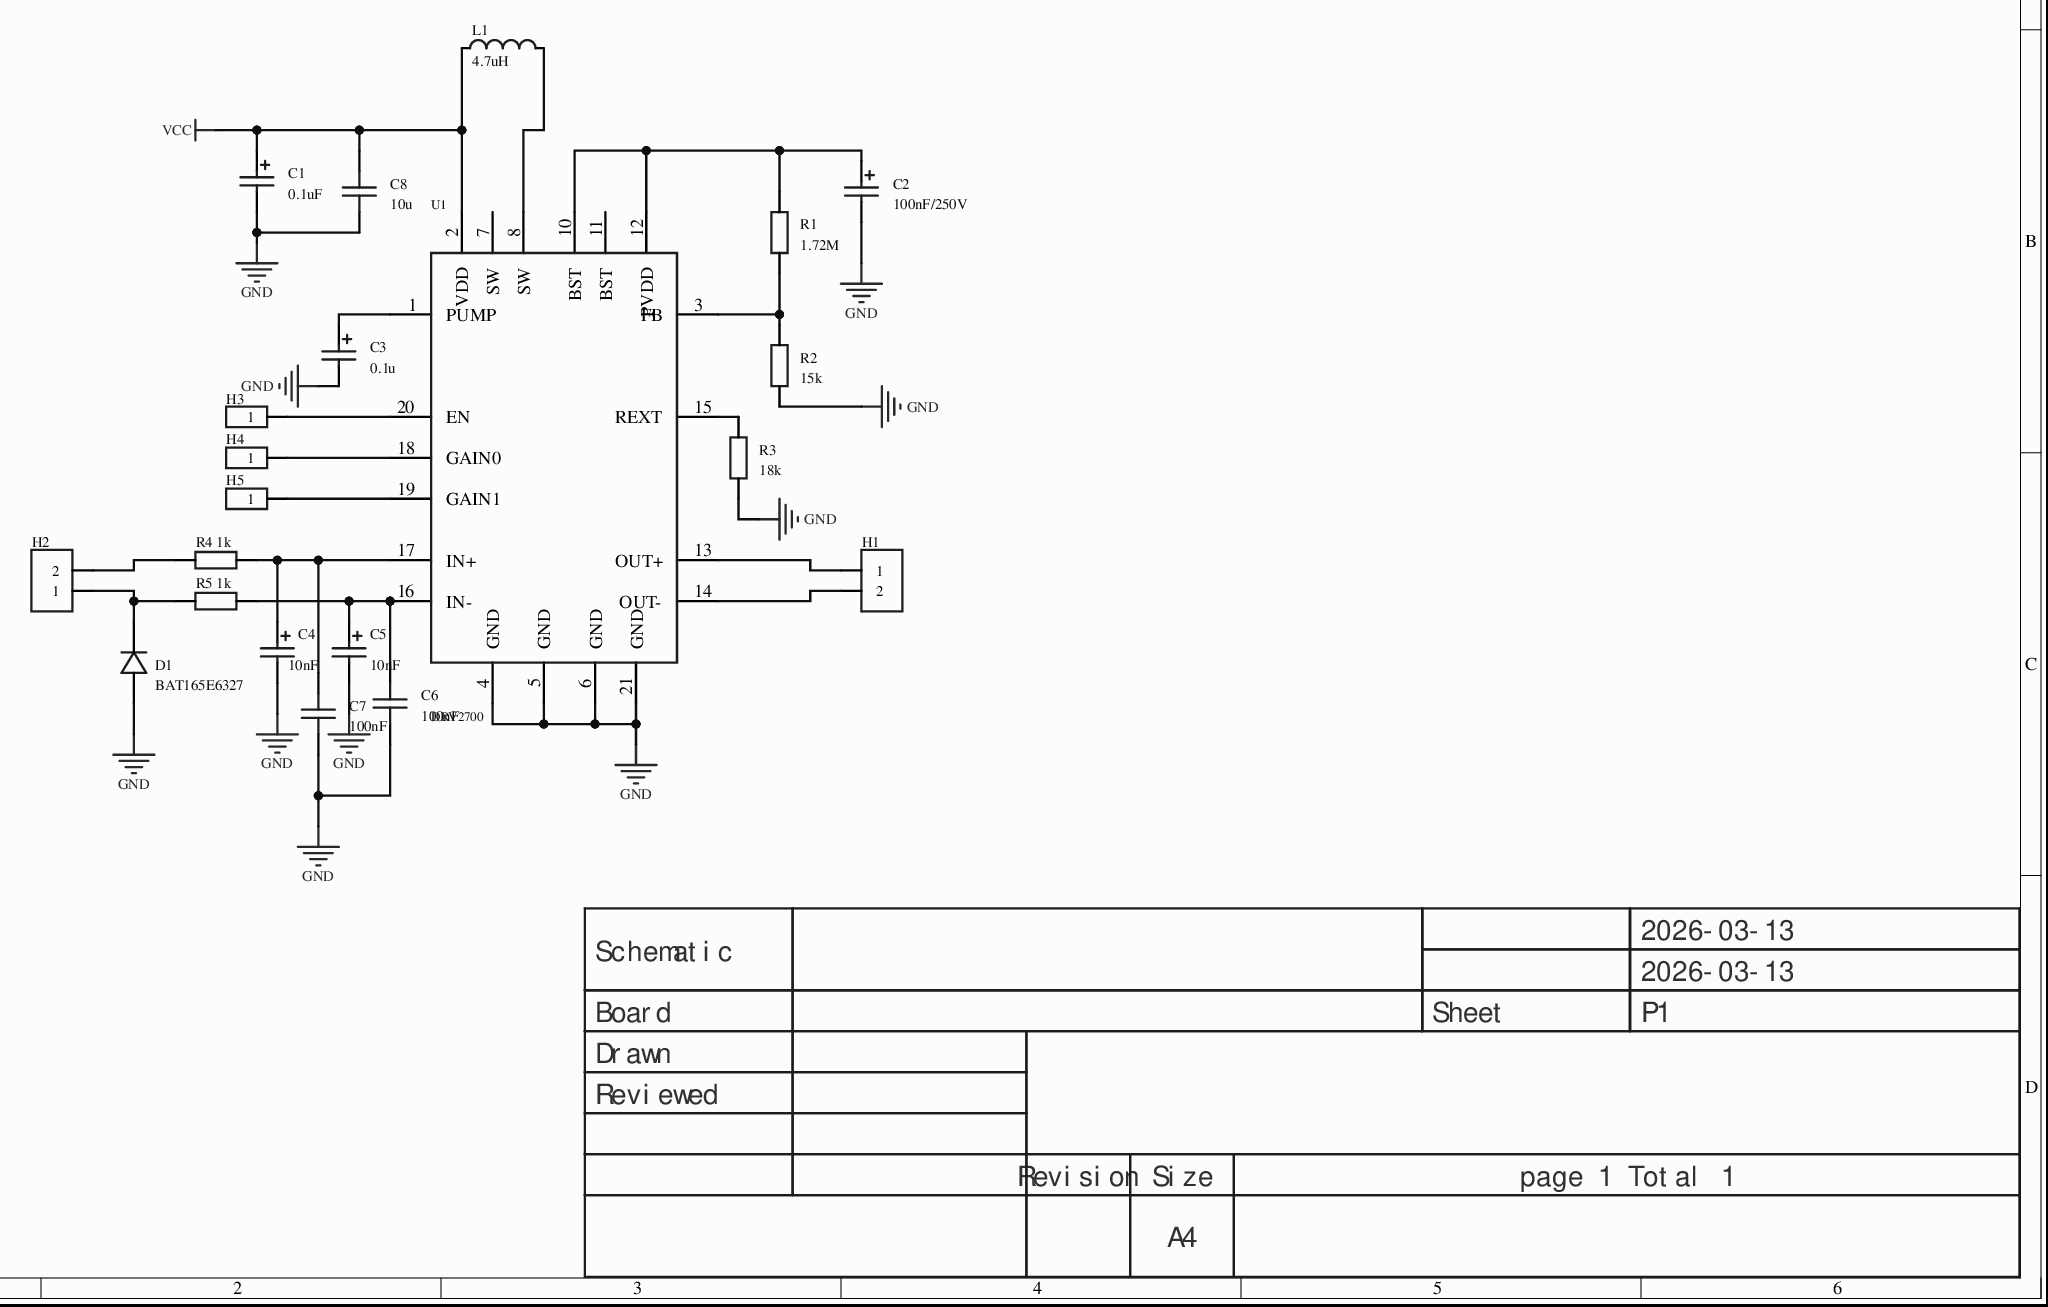
[diagram p0: MISC51187-3.schdoc]
# Altium project MISC51187-2.PrjPcb
1 sheet, 21 parts. Net scope: global (net labels, ports and power ports of the same name join across sheets).
Board file: MISC51187.pcbdoc

## Sheet MISC51187-3.schdoc
size 297 x 209 mm; Version: V1.0; @Project Name: MISC51187; @Update Date: 2026-03-13; @Create Date: 2026-03-13; @Board Name: MISC51187; @Create Time: 10:06:33; @Page Count: 1; @Page No: 1; @Schematic Name: MISC51187; @Update Time: 10:06:33; Size: A4

### Parts
C1  0.1uF  [C_Ele_SMD_3x5.4mm]
C2  100nF/250V  [C_Ele_SMD_3x5.4mm]
C3  0.1u  [C_Ele_SMD_3x5.4mm]
C4  10nF  [C_Ele_SMD_3x5.4mm]
C5  10nF  [C_Ele_SMD_3x5.4mm]
C6  100nF  [C0805]
C7  100nF  [C0805]
C8  10u  [C0805]
D1  BAT165E6327  [SOD-323_L1.8-W1.3-LS2.5-RD]
H1  (no value)  [HDR-TH_2P-P2.54-V-F]
H2  (no value)  [HDR-TH_2P-P2.54-V-F]
H3  (no value)  [HDR-TH_1P-V-M_XKB_X4611WV-01I-C28D40]
H4  (no value)  [HDR-TH_1P-V-M_XKB_X4611WV-01I-C28D40]
H5  (no value)  [HDR-TH_1P-V-M_XKB_X4611WV-01I-C28D40]
L1  4.7uH  [IND-SMD_L4.6-W4.1-A]
R1  1.72M  [Res_1W]
R2  15k  [Res_1W]
R3  18k  [Res_1/4W]
R4  1k  [Res_1/4W]
R5  1k  [Res_1/4W]
U1  DRV2700  [TI-RGP20-2700X2700TP_V]

### Nets
GND: C1.2 C2.2 C3.2 C4.2 C5.2 C6.1 C7.1 C8.1 D1.2(A) R2.1 R3.1 U1.4(GND) U1.5(GND) U1.6(GND) U1.21(GND)
VCC: C1.1 C8.2 L1.1 U1.2(VDD)
NetC2_1: C2.1 R1.2 U1.10(BST) U1.12(PVDD)
NetC3_1: C3.1 U1.1(PUMP)
NetC4_1: C4.1 C7.2 R4.2 U1.17(IN+)
NetC5_1: C5.1 C6.2 R5.2 U1.16(IN-)
NetD1_1: D1.1(C) H2.1 R5.1
NetH1_1: H1.1 U1.13(OUT+)
NetH1_2: H1.2 U1.14(OUT-)
NetH2_2: H2.2 R4.1
NetH3_1: H3.1 U1.20(EN)
NetH4_1: H4.1 U1.18(GAIN0)
NetH5_1: H5.1 U1.19(GAIN1)
NetL1_2: L1.2 U1.8(SW)
NetR1_1: R1.1 R2.2 U1.3(FB)
NetR3_2: R3.2 U1.15(REXT)

Not connected (* = marked no-connect by the designer): U1 7(SW)* 11(BST)*

### Notes on the sheet
- 2026-03-13
- Schematic
- Board
- Sheet
- P1
- Drawn
- Reviewed
- Revision
- Size
- A4
- page 1 Total 1

### Library data of the parts
C1-C5 = C_Ele_SMD_3x5.4mm: Symbol: CAP; 3D Model: 0132c3d3fdbf4fd987f710a97e7a5b5d0819f05c4eef4c71ace90d822a990e87; 3D Model Transform: 129.9,149.58,209.06,-90,0,0,0,0,0; AddInBom: yes; ModelName: CAP-SMD_BD3.0-L3.3-W3.3-H5.3; Device: C_Ele_SMD_3x5.4mm; Supplier Footprint: SMD,3x5.4mm; FootprintName: C_Ele_SMD_3x5.4mm; ConvertToPcb: yes
  C1: Value: 0.1uF
  C2: Value: 100nF/250V
  C3: Value: 0.1u
  C4 C5: Value: 10nF
C6-C8 = CAP_0805: Symbol: Capacitance; 3D Model: 1ba041120af144c991958decab20d2410819f05c4eef4c71ace90d822a990e87; 3D Model Transform: 78.74,51.181,0,0,0,0,0,0.0005,0; ConvertToPcb: yes; ModelName: C0805_L2.0-W1.3-H1.3; Device: CAP_0805; Supplier Footprint: 0805; FootprintName: C0805; AddInBom: yes
  C6 C7: Value: 100nF
  C8: Value: 10u
D1 = BAT165E6327: component BAT165E6327 compon Diode configuration: 1 single; Forward voltage (Vf): 740mV@750mA; DC reverse voltage (Vr): 40V; Rectifier current: 750mA;; Manufacturer: Infineon(英飞凌); Symbol: BAT165E6327HTSA1; Reverse Leakage Current (Ir): 50uA@40V; Non-Repetitive Peak Forward Surge Current: 2.5A; 3D Model: 7459fe65e23146c0a8d836e46a0add720819f05c4eef4c71ace90d822a990e87; 3D Model Transform: 104.3305,51.181,0,0,0,0,0,0,0; AddInBom: yes; Device: BAT165E6327; LCSC Part Name: 电压:40V 电流:750mA; Supplier Part: C151511; Manufacturer Part: BAT165E6327; Supplier Footprint: SOD-323; JLCPCB Part Class: Extended Part; Datasheet: https://item.szlcsc.com/datasheet/BAT165E6327/162851.html; Supplier: LCSC; Diode Configuration: 1 single; Voltage - Forward(Vf@If): 740mV@750mA; Voltage - DC Reverse(Vr): 40V; Current - Rectified: 750mA; FootprintName: SOD-323_L1.8-W1.3-LS2.5-RD; ConvertToPcb: yes; ModelName: SOD-323_L1.8-W1.3-LS2.5-RD
H1 H2 = HDR-F_2.54_1x2P: Symbol: Header-Female-2.54_1x2; 3D Model: a9450ef445564560a104363b9aacde4e0819f05c4eef4c71ace90d822a990e87; 3D Model Transform: 215.7476,98.425,0,0,0,0,0,0,-129.921; ConvertToPcb: yes; ModelName: HDR-TH_2P-P2.54-F-LI-1X2P; Device: HDR-F_2.54_1x2P; Supplier Part: C49661; Supplier Footprint: 插件; FootprintName: HDR-TH_2P-P2.54-V-F; AddInBom: yes
H3-H5 = HDR-M_2.54_1x1P: Symbol: HDR_1x1; 3D Model: 95857080d3cc4057a19a22ccce05e1710819f05c4eef4c71ace90d822a990e87; 3D Model Transform: 78.74,79.1337,0,0,0,0,0,0,-110.236; ConvertToPcb: yes; Device: HDR-M_2.54_1x1P; Supplier Part: C81276; Supplier Footprint: 插件; JLCPCB Part Class: Extended Part; FootprintName: HDR-TH_1P-V-M_XKB_X4611WV-01I-C28D40; AddInBom: yes; ModelName: HDR-TH_1P-V-M_XKB_X4611WV-01I-C28D40
L1 = SRG0420-4R7-M: component SRG0420-4R7-M comp Inductance: 4.7uH; Tolerance: ±20%; Rated current: 3A; Saturation current (Isat): 3.5A; Type: molded inductor;; Manufacturer: JIERR(捷而瑞); DC Resistance(DCR): 105mΩ; 3D Model: 3b00517e351145dc8b8e2e52a7e5ed2c0819f05c4eef4c71ace90d822a990e87; 3D Model Transform: 181.102,161.417,0,0,0,0,0,0,0; AddInBom: yes; ModelName: IND-SMD_L4.6-W4.1-H1.5; Symbol: SRG0420-4R7-M; Device: SRG0420-4R7-M; LCSC Part Name: 4.7μH ±20% 3.5A; Supplier Part: C53462918; Manufacturer Part: SRG0420-4R7-M; Supplier Footprint: SMD,4.6x4.1mm; JLCPCB Part Class: Extended Part; Datasheet: https://item.szlcsc.com/datasheet/SRG0420-4R7-M/56628163.html; Supplier: LCSC; Value: 4.7uH; Current Rating: 3A; Current - Saturation(Isat): 3.5A; Type: Molded inductor; FootprintName: IND-SMD_L4.6-W4.1-A; ConvertToPcb: yes
R1-R5 = Res_AXIAL-1W: Symbol: Resistor; 3D Model: f1f7cfb3d56f4763951150e77c261d090819f05c4eef4c71ace90d822a990e87; 3D Model Transform: 641.71,177.16,374,0,0,0,0,0,-190; ConvertToPcb: yes; ModelName: RES-TH_BD4.5-L11.5-P15.50-D0.8; Device: Res_AXIAL-1W; Supplier Footprint: 轴向引线; AddInBom: yes
  R1: Value: 1.72M; FootprintName: Res_1W
  R2: Value: 15k; FootprintName: Res_1W
  R3: Value: 18k; FootprintName: Res_1/4W
  R4 R5: Value: 1k; FootprintName: Res_1/4W
U1 = DRV2700: Symbol: DRV2700; Device: DRV2700; FootprintName: TI-RGP20-2700X2700TP_V